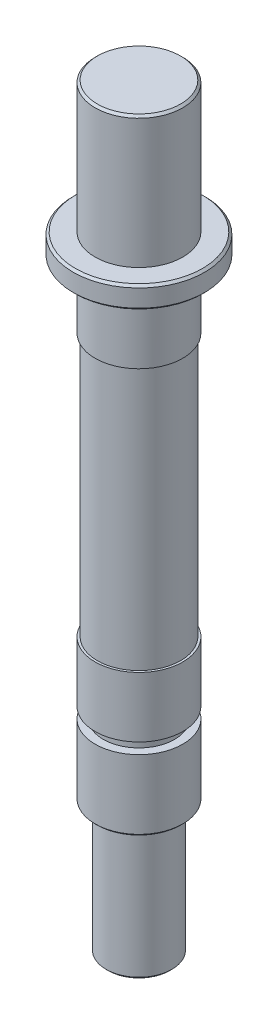
SolidWorks part; units mm, degrees
ref_plane "Front Plane" through (0, 0, 0) normal (0, 0, 1) x (1, 0, 0)
ref_plane "Top Plane" through (0, 0, 0) normal (0, 1, 0) x (1, 0, 0)
ref_plane "Right Plane" through (0, 0, 0) normal (1, 0, 0) x (0, 0, -1)
sketch "Sketch1" plane through (0, 0, 0) normal (0, 1, 0) x (1, 0, 0)
  circle A0 centre (0, 0) radius 4
  dimension "D1" = 8
extrude "Boss-Extrude1" add sketch "Sketch1" along normal blind 43
cosmetic thread "Cosmetic Thread1" parameters "D1"=6, "D2"=6.917
sketch "Sketch2" plane through (0, 43, 0) normal (0, 1, 0) x (1, 0, 0)
  circle A0 centre (0, 0) radius 6
  dimension "D1" = 12
extrude "Boss-Extrude2" add sketch "Sketch2" along normal blind 2
sketch "Sketch10" plane through (0, 45, 0) normal (0, 1, 0) x (1, 0, 0)
  circle A0 centre (0, 0) radius 4
  dimension "D1" = 8
extrude "Boss-Extrude4" add sketch "Sketch10" along normal blind 12
sketch "Sketch8" plane through (0, 0, 0) normal (0, 0, 1) x (1, 0, 0)
  line L0 (0, 0) -> (0, 78.0455) construction
  line L2 (-4, 43) -> (4, 43) construction
  line L3 (3.8, 37) -> (7.8857, 37)
  line L4 (3.8, 37) -> (3.8, 13)
  line L5 (3.8, 13) -> (7.8857, 13)
  line L6 (7.8857, 37) -> (7.8857, 13)
  line L7 (-4, 0) -> (4, 0) construction
  line L8 (3.25, 7.5) -> (7.1798, 7.5)
  line L9 (3.25, 7.5) -> (3.25, 6.5)
  line L10 (3.25, 6.5) -> (7.1798, 6.5)
  line L11 (7.1798, 7.5) -> (7.1798, 6.5)
  dimension "D1" = 7.6
  dimension "D2" = 6
  dimension "D3" = 24
  dimension "D4" = 5.5
  dimension "D5" = 1
  dimension "D6" = 6.5
revolve "Cut-Revolve1" cut sketch "Sketch8" angle 360 about L0
sketch "Sketch9" plane through (0, 0, 0) normal (0, -1, 0) x (1, 0, 0)
  circle A0 centre (0, 0) radius 3
  dimension "D1" = 6
extrude "Boss-Extrude3" add sketch "Sketch9" along normal blind 12
chamfer "Chamfer1" distance 0.2 angle 45 5 edges at (0, -12, -3) (0, 0, 4) (0, 43, 6) (0, 57, 4) (0, 45, 6)
